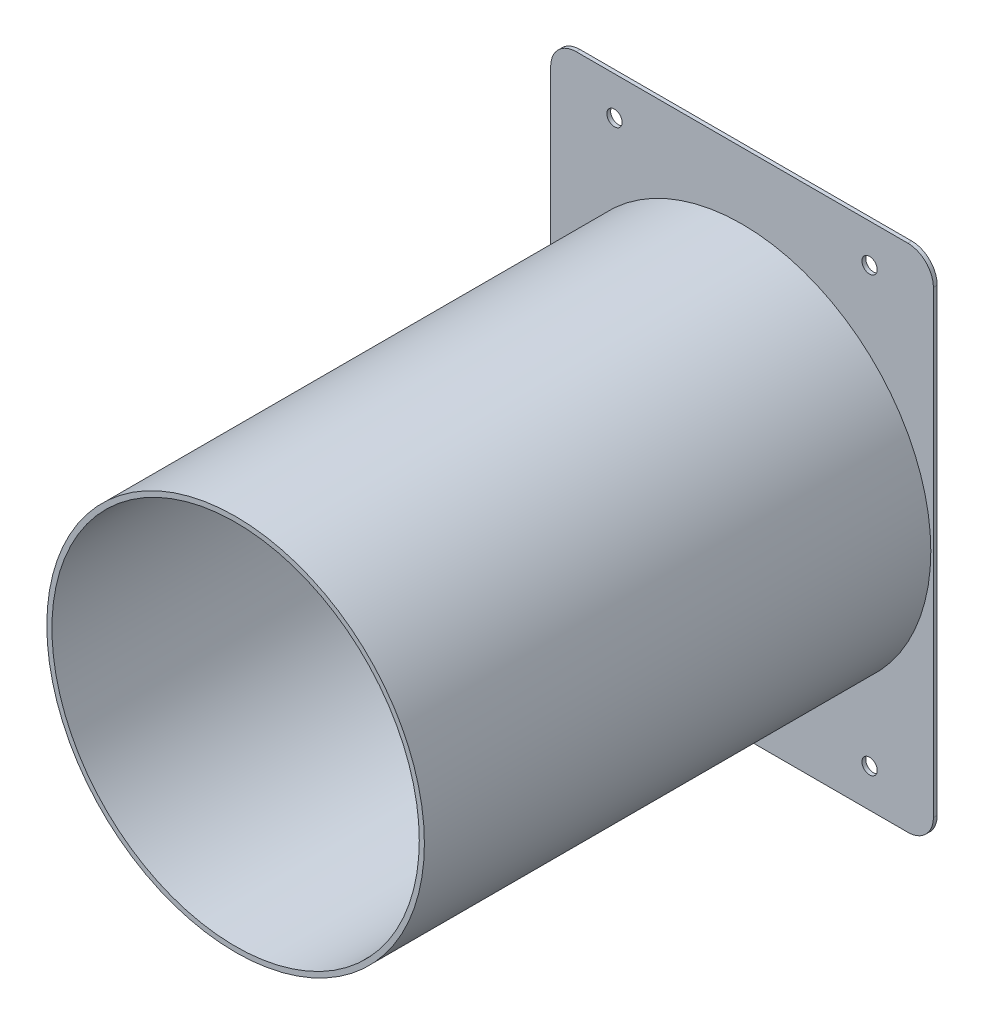
SolidWorks part; units mm, degrees
material "SUS304"
ref_plane "前视基准面" through (0, 0, 0) normal (0, 0, 1) x (1, 0, 0)
ref_plane "上视基准面" through (0, 0, 0) normal (0, 1, 0) x (1, 0, 0)
ref_plane "右视基准面" through (0, 0, 0) normal (1, 0, 0) x (0, 0, -1)
sketch "草图1" plane through (0, 0, 0) normal (0, 0, 1) x (1, 0, 0)
  circle A0 centre (0, 0) radius 74
  circle A1 centre (0, 0) radius 72
  dimension "D1" = 148
  dimension "D2" = 144
extrude "凸台-拉伸1" add sketch "草图1" along normal blind 200
sketch "草图2" plane through (0, 0, 0) normal (0, 0, -1) x (-1, 0, 0)
  line L1 (-75, -100) -> (75, -100)
  line L2 (-75, -100) -> (-75, 100)
  line L3 (-75, 100) -> (75, 100)
  line L4 (75, -100) -> (75, 100)
  line L5 (-75, -100) -> (75, 100) construction
  line L6 (-75, 100) -> (75, -100) construction
  circle A0 centre (0, 0) radius 74
  circle A1 centre (0, 0) radius 74 construction
  point P0 (0, 0)
  dimension "D1" = 200
  dimension "D2" = 150
extrude "凸台-拉伸2" add sketch "草图2" against normal blind 1.5
fillet "圆角1" radius 10 4 edges at (75, 100, 0.75) (75, -100, 0.75) (-75, -100, 0.75) (-75, 100, 0.75)
hole_wizard "Ø6.0 (6) 直径孔1" positions "草图3" profile "草图4" hole size "Ø6.0" standard "ISO" end condition through all
sketch "草图3" plane through (0, 0, 1.5) normal (0, 0, 1) x (1, 0, 0)
  line L1 (-50, -85) -> (50, -85)
  line L2 (-50, -85) -> (-50, 85)
  line L3 (-50, 85) -> (50, 85)
  line L4 (50, -85) -> (50, 85)
  line L5 (-50, -85) -> (50, 85)
  point P0 (-50, -85)
  point P2 (-50, 85)
  point P4 (50, 85)
  point P6 (50, -85)
  dimension "D1" = 170
  dimension "D2" = 100
sketch "草图4" plane through (-50, -85, 1.5) normal (1, 0, 0) x (0, -1, 0)
  line L0 (0, 0) -> (0, 1.5)
  line L1 (0, 1.5) -> (3, 1.5)
  line L2 (3, 1.5) -> (3, 0)
  line L5 (3, 0) -> (0, 0)
  line L11 (0, -6.35) -> (0, 107.95) construction
  dimension "通孔孔直径" = 6
  dimension "通孔孔深度" = 1.5
